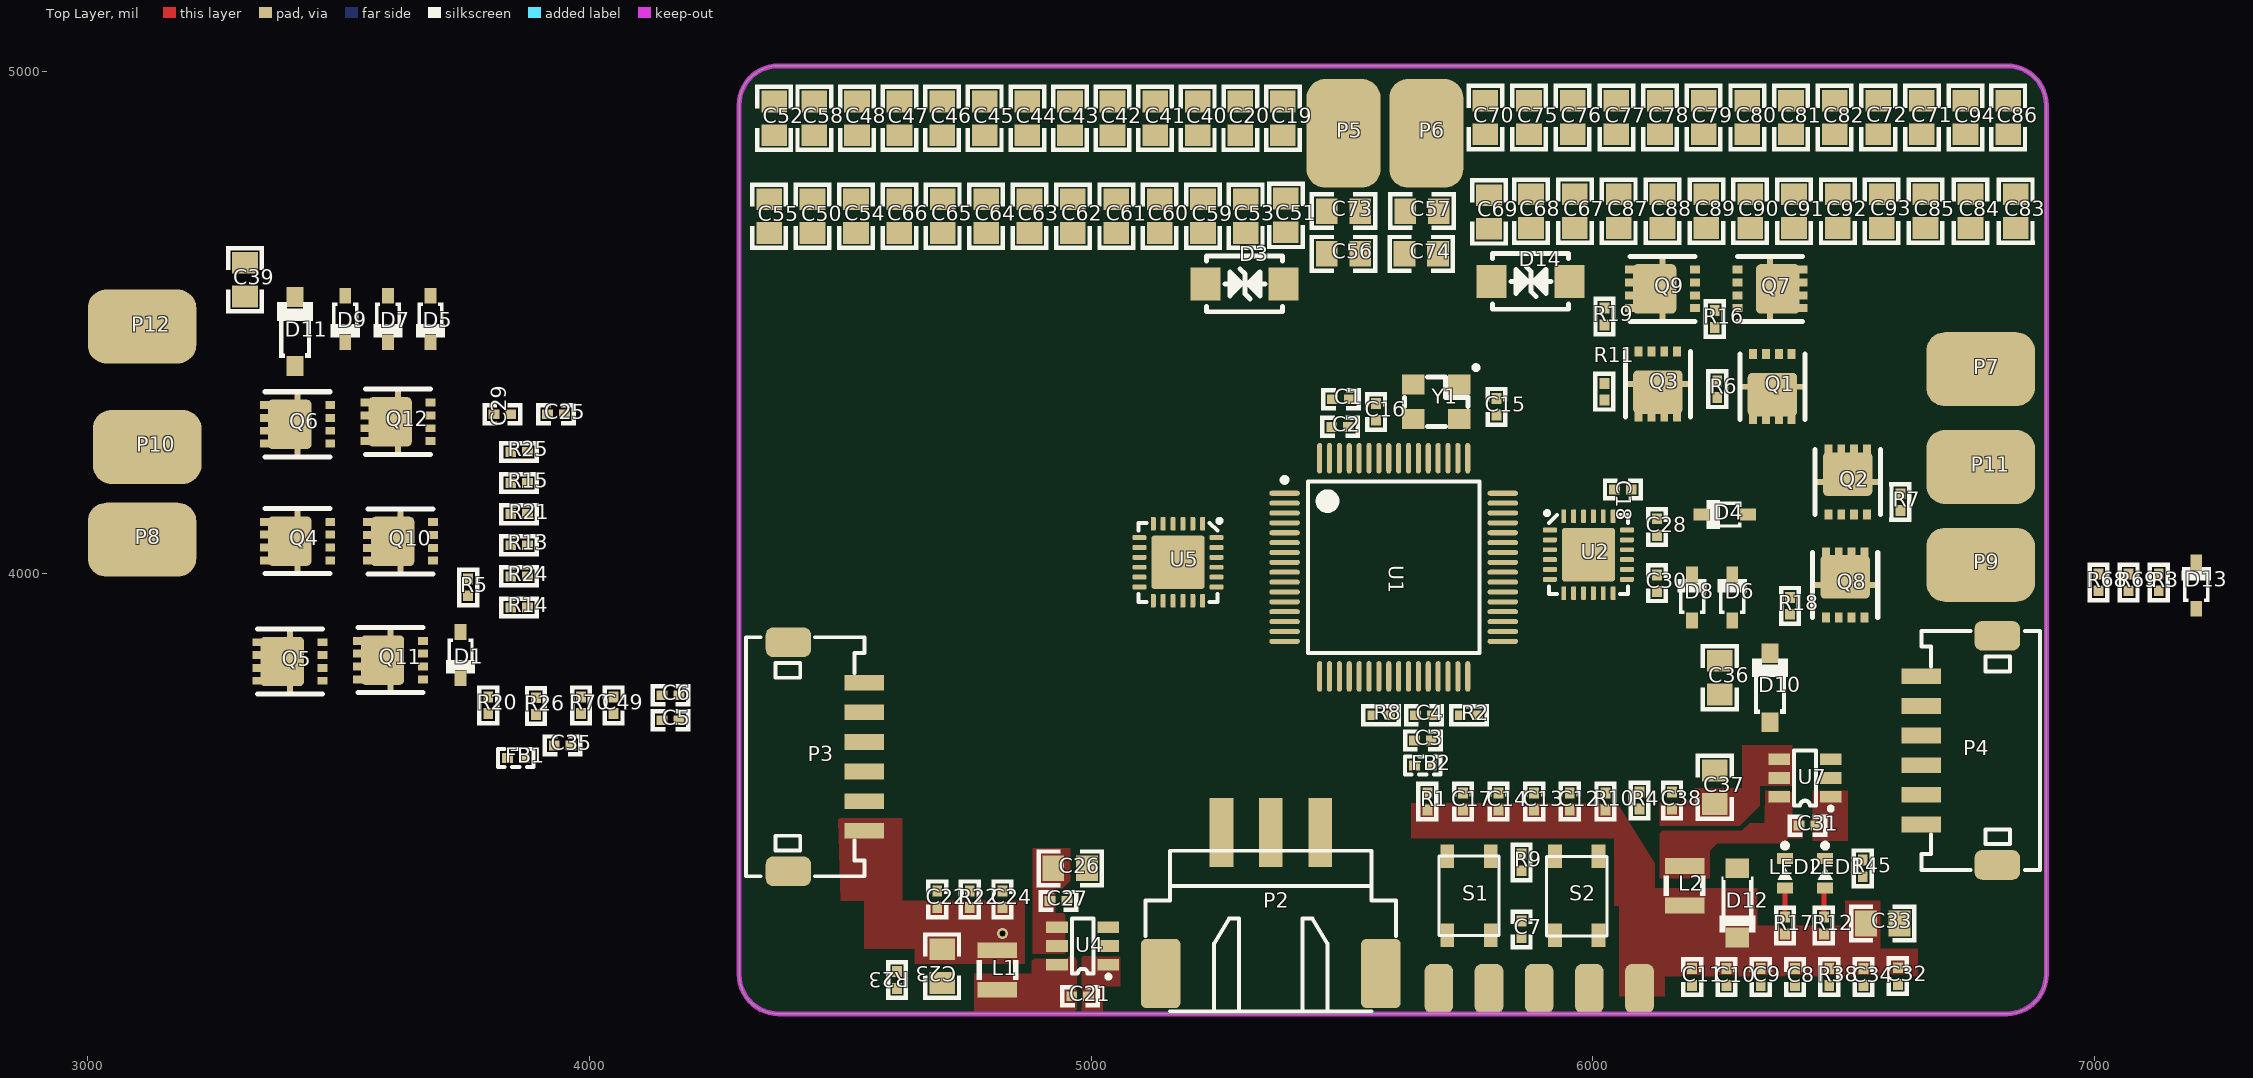
[diagram p0: Top Layer view]
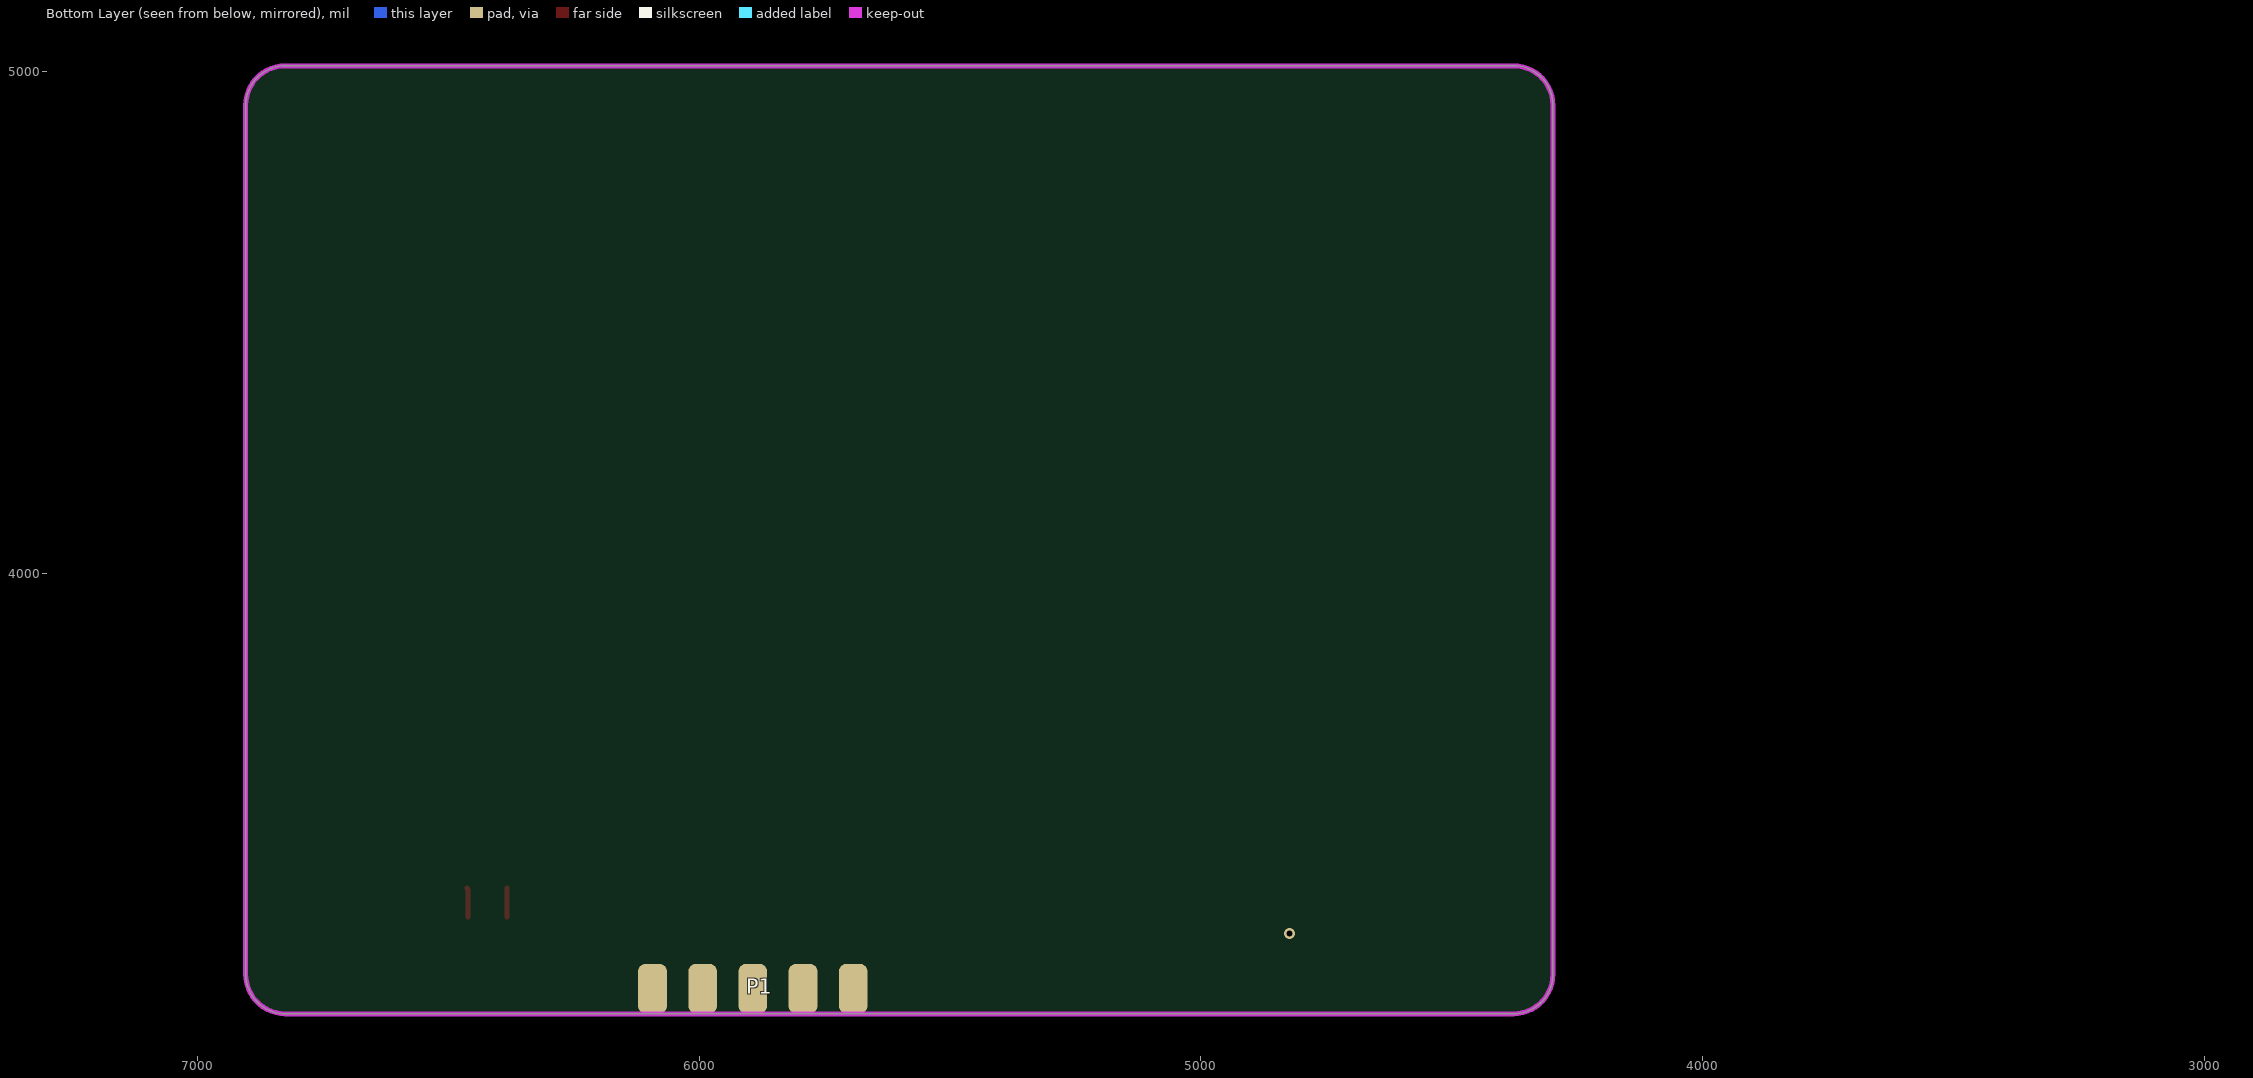
[diagram p1: Bottom Layer view, seen from below]
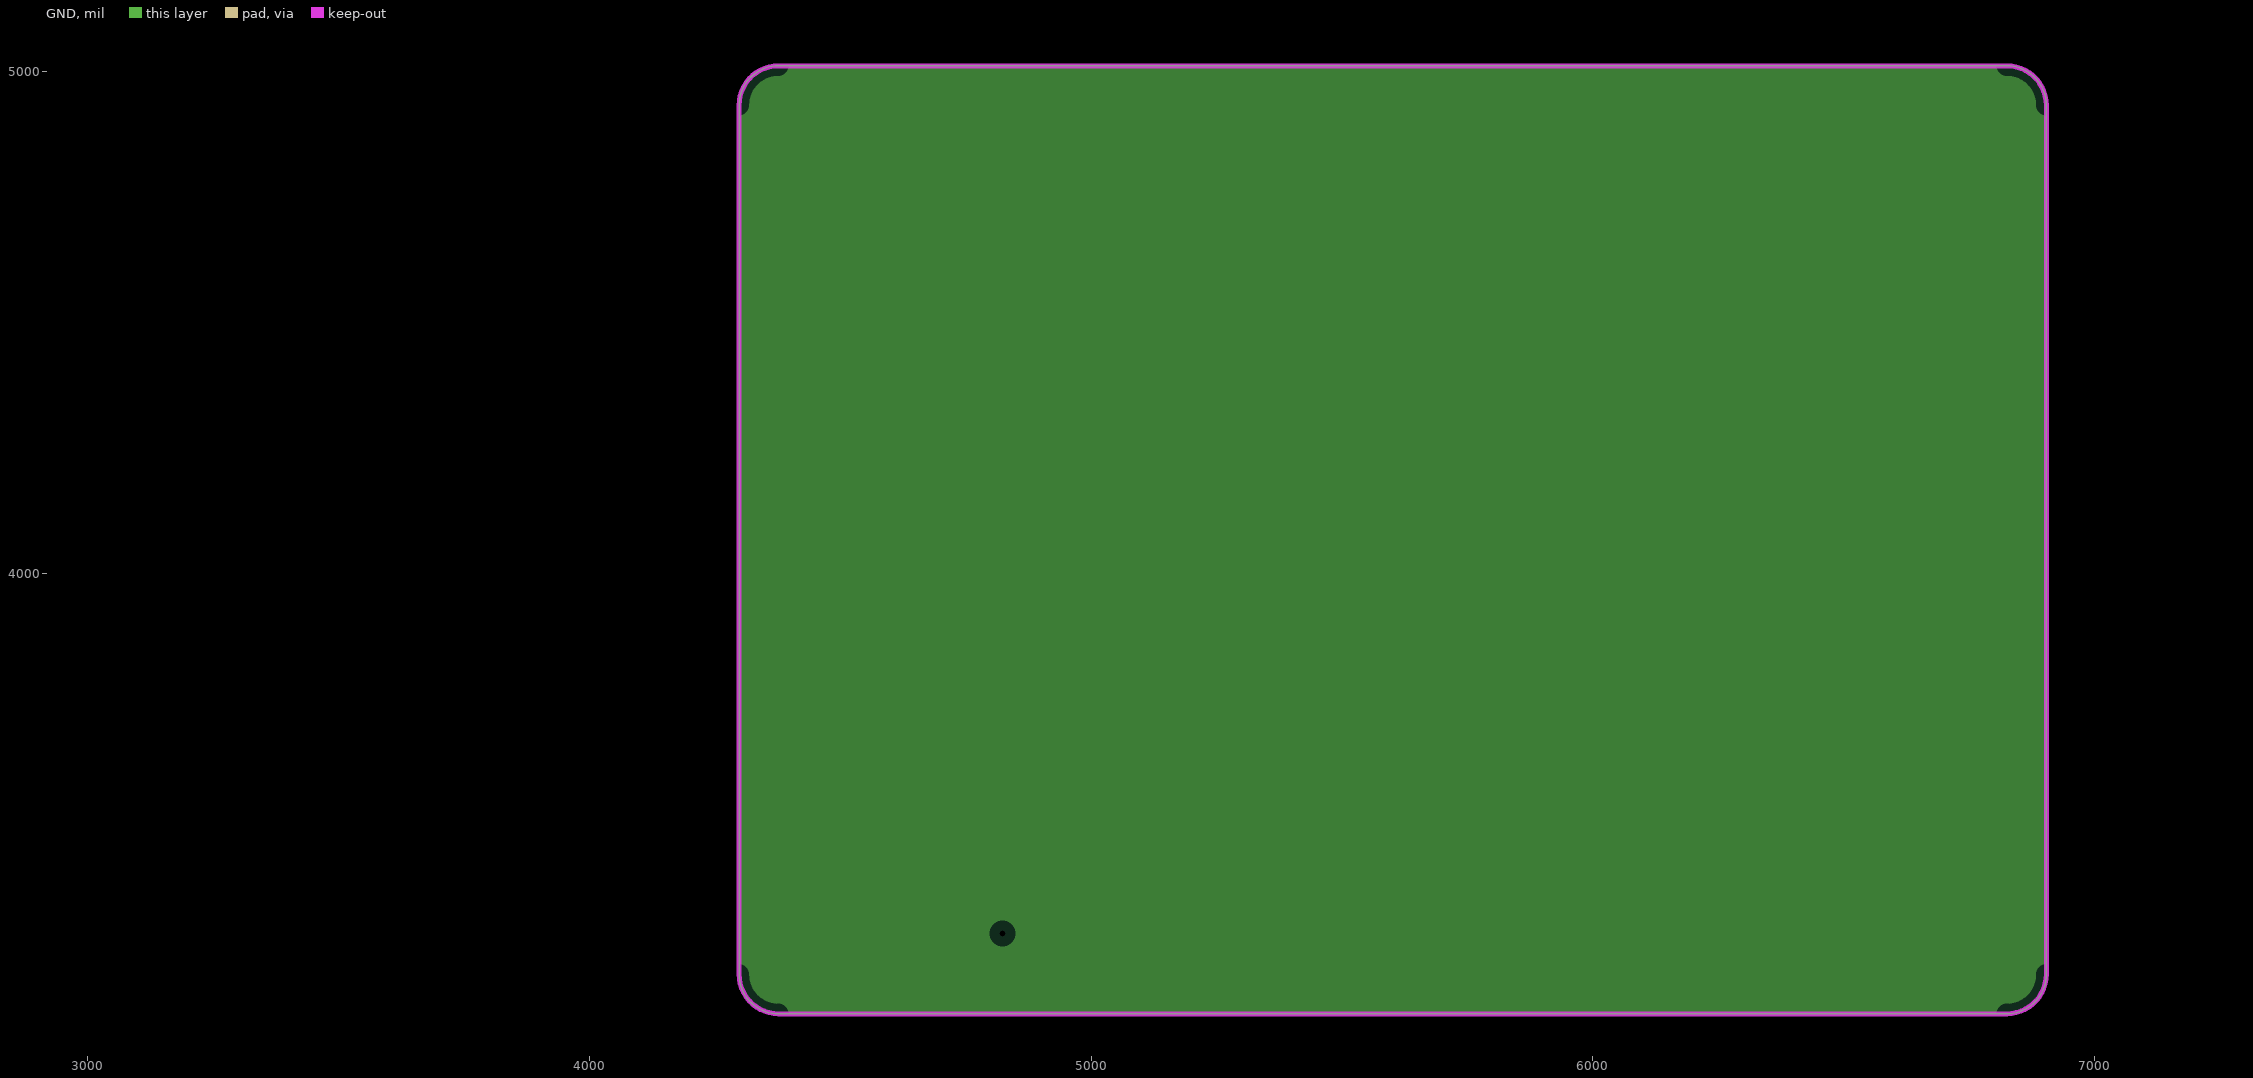
[diagram p2: GND, clearances drawn from the general rule]
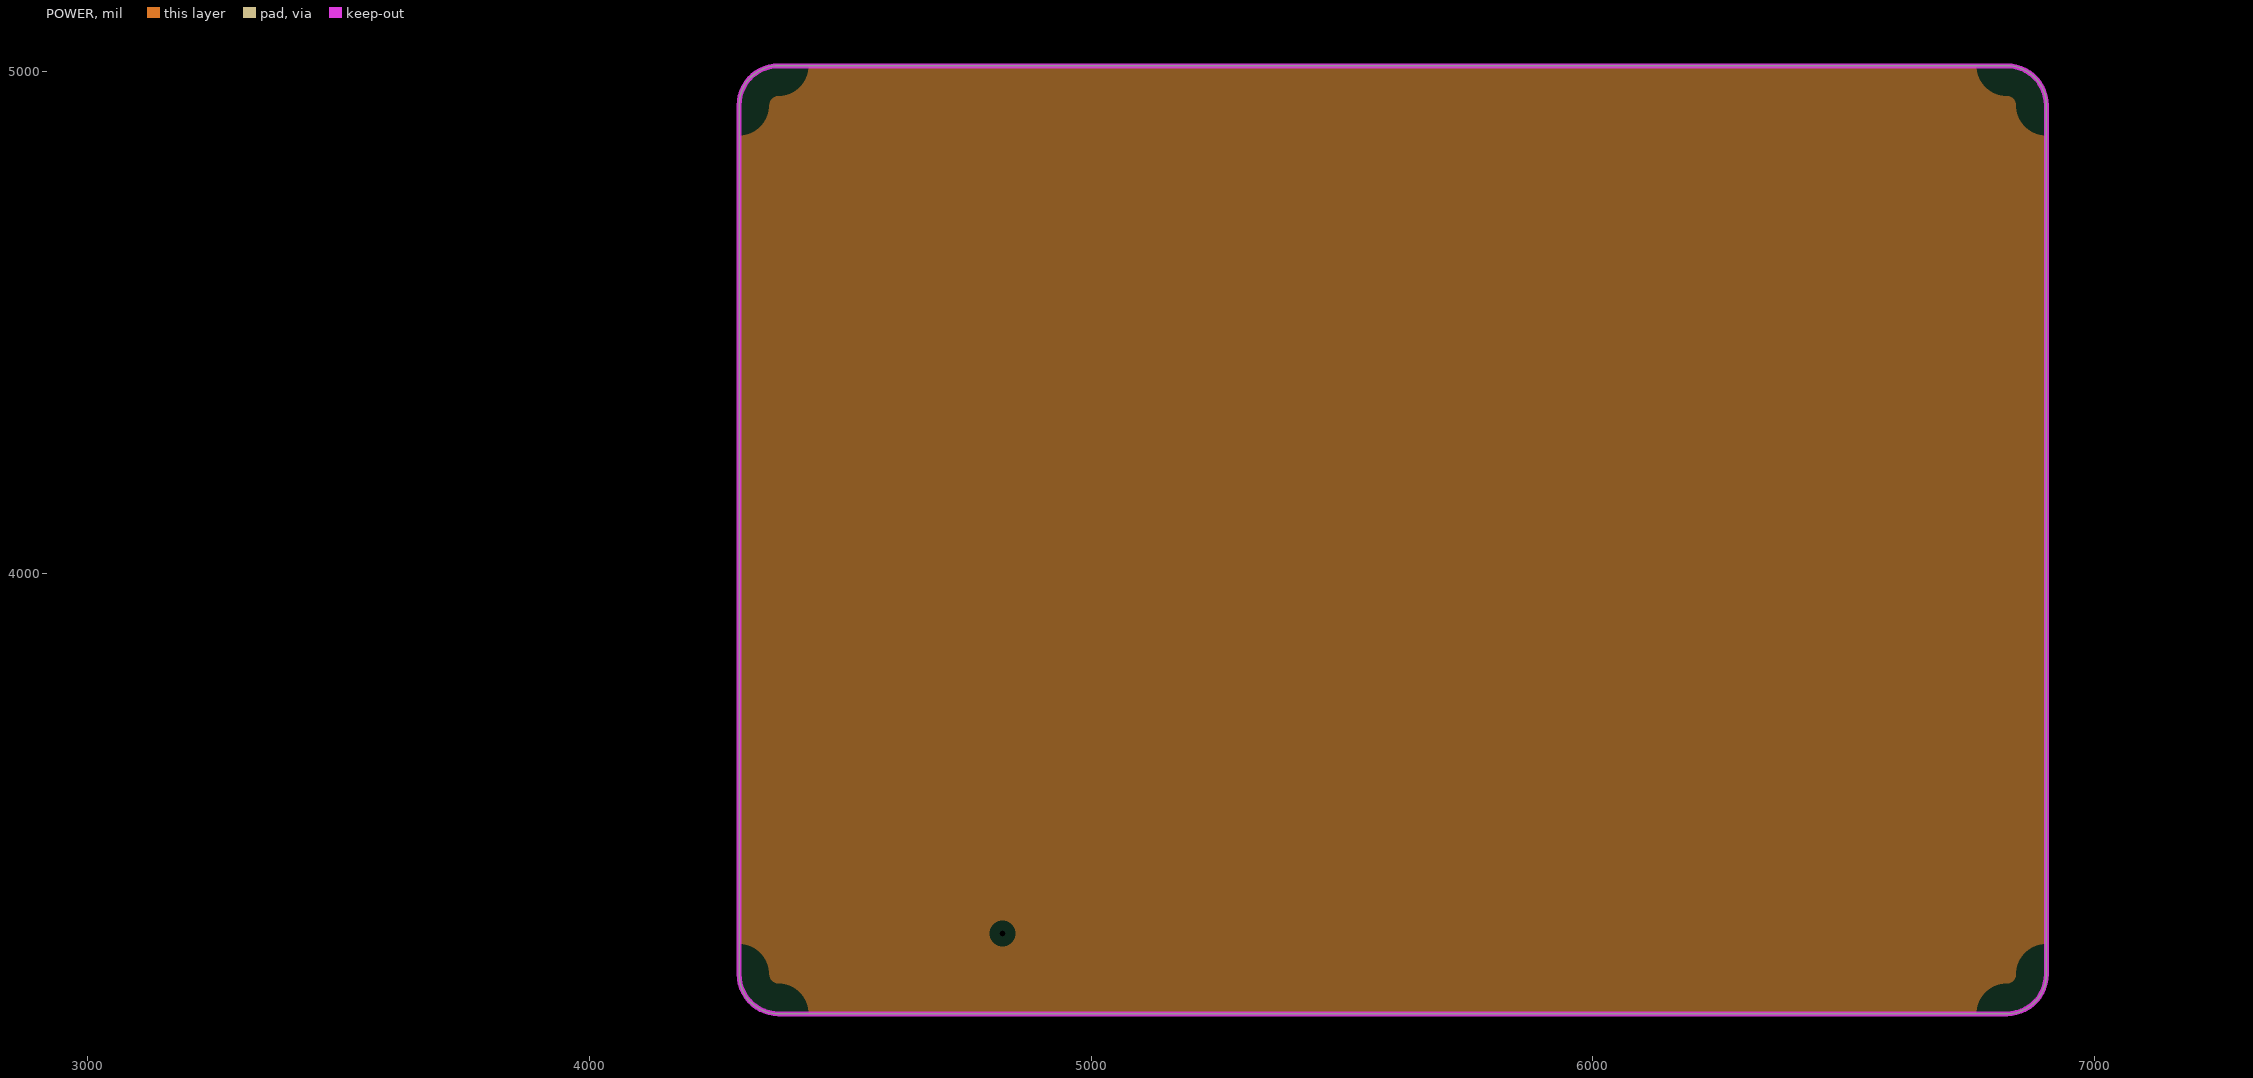
[diagram p3: POWER, clearances drawn from the general rule]
# Altium PCB MISC49862.pcbdoc
Units mil, origin at the board's own origin, x right, y up, seen from the top; angles counter-clockwise.
Board outline 2605.91 x 1889.76 mil, 4 copper layers (Top Layer, GND, POWER, Bottom Layer), stack 23.756 mil thick; 176 components, 102 nets, 585 pads, 1 vias.

## Layer stack, top to bottom
Top Solder Mask Layer: solder mask 0.4, Solder Resist, Dk 3.5
Top Layer: signal copper 1.4
Dielectric 3: surface 2.8, PP-006, Dk 4.1
GND: plane copper 1.378
Dielectric 2: surface 2.8, PP-006, Dk 4.1
POWER: plane copper 1.378
Dielectric 1: surface 12.6, FR-4, Dk 4.8
Bottom Layer: signal copper 1.4
Bottom Solder Mask Layer: solder mask 0.4, Solder Resist, Dk 3.5

## Board outline
6825.43,3122.38 4377.01,3122.38 cw(c4377.01,3201.12) 4298.27,3201.12 4298.27,4933.4 cw(c4377.01,4933.4) 4377.01,5012.14 6825.43,5012.14 cw(c6825.43,4933.4) 6904.17,4933.4 6904.17,3201.12 cw(c6825.43,3201.12)

## Design rules (kind name [scope] priority, off if disabled: settings)
HoleToHoleClearance Clearance_1 [All] p1 off: gap=11.8 allowstackedmicrovias=TRUE
HoleToHoleClearance Clearance [All] p2 off: gap=11.8 allowstackedmicrovias=TRUE
HoleToHoleClearance Width [All] p3 off: gap=120 allowstackedmicrovias=TRUE
HoleToHoleClearance DiffPairsRouting [All] p4 off: gap=15 allowstackedmicrovias=TRUE
HoleToHoleClearance RoutingVias [All] p5 off: gap=25 allowstackedmicrovias=TRUE
HoleToHoleClearance PlaneConnect [All] p6 off: gap=1 allowstackedmicrovias=TRUE
HoleToHoleClearance PolygonConnect [All] p7 off: gap=1 allowstackedmicrovias=TRUE
HoleToHoleClearance SolderMaskExpansion [All] p8 off: gap=4 allowstackedmicrovias=TRUE
HoleToHoleClearance PasteMaskExpansion [All] p9 off: gap=11.8 allowstackedmicrovias=TRUE
HoleToHoleClearance [All] p10: gap=10 allowstackedmicrovias=TRUE

## Components (designator, comment, footprint, x,y, rotation, side; value= is the part's Value field where it differs from the comment)
C1 "4.7uF 10V X5R" CAPC1005[0402]S-N 5498.27,4347.38 r0 top
C2 "100nF 16V X7R" CAPC1005[0402]S-N 5496.54,4292.38 r0 top
C3 "4.7uF 10V X5R" CAPC1005[0402]S-N 5661.54,3667.38 r180 top
C4 "100nF 16V X7R" CAPC1005[0402]S-N 5663.27,3717.38 r0 top
C5 "2.2uF 10V X5R" CAPC1005[0402]S-N 4161.54,3707.38 r0 top
C6 "100nF 16V X7R" CAPC1005[0402]S-N 4161.54,3757.38 r0 top
C7 "100nF 16V X7R" CAPC1005[0402]S-N 5858.27,3290.65 r270 top
C8 "4.7uF 10V X5R" CAPC1005[0402]S-N 6403.26,3195.65 r90 top
C9 "4.7uF 10V X5R" CAPC1005[0402]S-N 6334.93,3195.68 r270 top
C10 "100nF 16V X7R" CAPC1005[0402]S-N 6266.59,3195.65 r90 top
C11 "100nF 16V X7R" CAPC1005[0402]S-N 6198.27,3195.69 r270 top
C12 "4.7uF 10V X5R" CAPC1005[0402]S-N 5954.27,3545.65 r270 top
C13 "100nF 16V X7R" CAPC1005[0402]S-N 5883.27,3545.65 r270 top
C14 "4.7uF 10V X5R" CAPC1005[0402]S-N 5812.27,3545.65 r270 top
C15 "10pF 50V C0G" CAPC1005[0402]S-N 5808.27,4332.38 r270 top
C16 "10pF 50V C0G" CAPC1005[0402]S-N 5568.27,4322.38 r270 top
C17 "100nF 16V X7R" CAPC1005[0402]S-N 5741.27,3545.65 r270 top
C18 "4.7uF 10V X5R" CAPC1005[0402]S-N 6060,4167.38 r180 top
C19 "22uF 25V X5R" CAPC2012[0805]S-N 5382.43,4907.36 r90 top
C20 "22uF 25V X5R" CAPC2012[0805]S-N 5297.52,4907.38 r90 top
C21 "100nF 16V X7R" CAPC1005[0402]S-N 4978.27,3157.38 r180 top
C22 "220pF 50V X7R" CAPC1005[0402]S-N 4693.27,3350.65 r270 top
C23 "22uF 25V X5R" CAPC2012[0805]S-N 4703.27,3217.38 r90 top
C24 "100nF 16V X7R" CAPC1005[0402]S-N 4823.27,3350.65 r270 top
C25 "4.7uF 10V X5R" CAPC1005[0402]S-N 3933.27,4317.38 r0 top
C26 "22uF 25V X5R" CAPC2012[0805]S-N 4958.27,3412.38 r180 top
C27 "100nF 16V X7R" CAPC1005[0402]S-N 4935,3347.38 r180 top
C28 "4.7uF 10V X5R" CAPC1005[0402]S-N 6128.27,4092.38 r270 top
C29 "4.7uF 10V X5R" CAPC1005[0402]S-N 3826.54,4317.38 r0 top
C30 "4.7uF 10V X5R" CAPC1005[0402]S-N 6128.27,3980.65 r90 top
C31 "100nF 16V X7R" CAPC1005[0402]S-N 6428.27,3497.38 r180 top
C32 "220pF 50V X7R" CAPC1005[0402]S-N 6608.27,3197.38 r90 top
C33 "22uF 25V X5R" CAPC2012[0805]S-N 6578.27,3302.38 r180 top
C34 "100nF 16V X7R" CAPC1005[0402]S-N 6539.93,3195.65 r90 top
C35 "4.7uF 10V X5R" CAPC1005[0402]S-N 3946.54,3657.38 r0 top
C36 "22uF 25V X5R" CAPC2012[0805]S-N 6253.27,3792.38 r270 top
C37 "22uF 25V X5R" CAPC2012[0805]S-N 6243.27,3573.91 r270 top
C38 "100nF 16V X7R" CAPC1005[0402]S-N 6158.27,3547.38 r270 top
C39 "22uF 25V X5R" CAPC2012[0805]S-N 3313.27,4585.84 r90 top
C40 "22uF 25V X5R" CAPC2012[0805]S-N 5212.6,4907.36 r90 top
C41 "22uF 25V X5R" CAPC2012[0805]S-N 5127.68,4907.38 r90 top
C42 "22uF 25V X5R" CAPC2012[0805]S-N 5042.77,4907.36 r90 top
C43 "22uF 25V X5R" CAPC2012[0805]S-N 4957.85,4907.38 r90 top
C44 "22uF 25V X5R" CAPC2012[0805]S-N 4872.94,4907.37 r90 top
C45 "22uF 25V X5R" CAPC2012[0805]S-N 4788.02,4907.38 r90 top
C46 "22uF 25V X5R" CAPC2012[0805]S-N 4703.12,4907.36 r90 top
C47 "22uF 25V X5R" CAPC2012[0805]S-N 4618.18,4907.36 r90 top
C48 "22uF 25V X5R" CAPC2012[0805]S-N 4533.27,4907.36 r90 top
C49 "100nF 16V X7R" CAPC1005[0402]S-N 4048.27,3737.38 r270 top
C50 "22uF 25V X5R" CAPC2012[0805]S-N 4444.77,4712.38 r270 top
C51 "22uF 25V X5R" CAPC2012[0805]S-N 5388.27,4713.91 r270 top
C52 "22uF 25V X5R" CAPC2012[0805]S-N 4368.27,4907.38 r90 top
C53 "22uF 25V X5R" CAPC2012[0805]S-N 5308.27,4712.38 r270 top
C54 "22uF 25V X5R" CAPC2012[0805]S-N 4531.28,4712.38 r270 top
C55 "22uF 25V X5R" CAPC2012[0805]S-N 4358.27,4712.38 r270 top
C56 "22uF 25V X5R" CAPC2012[0805]S-N 5503.27,4637.38 r0 top
C57 "22uF 25V X5R" CAPC2012[0805]S-N 5659.8,4722.38 r180 top
C58 "22uF 25V X5R" CAPC2012[0805]S-N 4448.27,4907.36 r90 top
C59 "22uF 25V X5R" CAPC2012[0805]S-N 5223.27,4712.38 r270 top
C60 "22uF 25V X5R" CAPC2012[0805]S-N 5136.77,4712.38 r270 top
C61 "22uF 25V X5R" CAPC2012[0805]S-N 5050.28,4712.38 r270 top
C62 "22uF 25V X5R" CAPC2012[0805]S-N 4963.78,4712.38 r270 top
C63 "22uF 25V X5R" CAPC2012[0805]S-N 4877.28,4712.38 r270 top
C64 "22uF 25V X5R" CAPC2012[0805]S-N 4790.76,4712.38 r270 top
C65 "22uF 25V X5R" CAPC2012[0805]S-N 4704.28,4712.38 r270 top
C66 "22uF 25V X5R" CAPC2012[0805]S-N 4617.77,4712.38 r270 top
C67 "22uF 25V X5R" CAPC2012[0805]S-N 5964.5,4722.4 r90 top
C68 "22uF 25V X5R" CAPC2012[0805]S-N 5877.13,4722.35 r90 top
C69 "22uF 25V X5R" CAPC2012[0805]S-N 5793.27,4720.84 r90 top
C70 "22uF 25V X5R" CAPC2012[0805]S-N 5785.99,4908.91 r270 top
C71 "22uF 25V X5R" CAPC2012[0805]S-N 6656.24,4908.91 r270 top
C72 "22uF 25V X5R" CAPC2012[0805]S-N 6569.22,4908.91 r270 top
C73 "22uF 25V X5R" CAPC2012[0805]S-N 5503.27,4722.38 r180 top
C74 "22uF 25V X5R" CAPC2012[0805]S-N 5658.27,4637.38 r0 top
C75 "22uF 25V X5R" CAPC2012[0805]S-N 5873,4908.91 r270 top
C76 "22uF 25V X5R" CAPC2012[0805]S-N 5960.03,4908.91 r270 top
C77 "22uF 25V X5R" CAPC2012[0805]S-N 6047.06,4908.91 r270 top
C78 "22uF 25V X5R" CAPC2012[0805]S-N 6134.07,4908.91 r270 top
C79 "22uF 25V X5R" CAPC2012[0805]S-N 6221.11,4908.91 r270 top
C80 "22uF 25V X5R" CAPC2012[0805]S-N 6308.14,4908.91 r270 top
C81 "22uF 25V X5R" CAPC2012[0805]S-N 6395.16,4908.91 r270 top
C82 "22uF 25V X5R" CAPC2012[0805]S-N 6482.19,4908.91 r270 top
C83 "22uF 25V X5R" CAPC2012[0805]S-N 6843.27,4722.38 r90 top
C84 "22uF 25V X5R" CAPC2012[0805]S-N 6753.27,4722.38 r90 top
C85 "22uF 25V X5R" CAPC2012[0805]S-N 6663.27,4722.39 r90 top
C86 "22uF 25V X5R" CAPC2012[0805]S-N 6828.27,4908.91 r270 top
C87 "22uF 25V X5R" CAPC2012[0805]S-N 6051.83,4722.38 r90 top
C88 "22uF 25V X5R" CAPC2012[0805]S-N 6139.18,4722.37 r90 top
C89 "22uF 25V X5R" CAPC2012[0805]S-N 6226.52,4722.37 r90 top
C90 "22uF 25V X5R" CAPC2012[0805]S-N 6313.87,4722.38 r90 top
C91 "22uF 25V X5R" CAPC2012[0805]S-N 6401.22,4722.38 r90 top
C92 "22uF 25V X5R" CAPC2012[0805]S-N 6488.57,4722.38 r90 top
C93 "22uF 25V X5R" CAPC2012[0805]S-N 6575.92,4722.38 r90 top
C94 "22uF 25V X5R" CAPC2012[0805]S-N 6743.27,4908.9 r270 top
D1 "B5819WS" SOD-323 3743.27,3837.38 r270 top
D3 "SMAJ16CA" SMA[DO-214AC]-Bi 5305.93,4577.38 r180 top
D4 "B5819WS" SOD-323 6263.27,4117.38 r180 top
D5 "B5819WS" SOD-323 3683.27,4507.38 r270 top
D6 "B5819WS" SOD-323 6278.27,3952.38 r90 top
D7 "B5819WS" SOD-323 3598.27,4507.38 r270 top
D8 "B5819WS" SOD-323 6198.27,3952.38 r90 top
D9 "B5819WS" SOD-323 3513.27,4507.38 r270 top
D10 "BZT52C15" SOD-123-L 6353.27,3772.38 r90 top
D11 "BZT52C15" SOD-123-L 3413.27,4482.38 r90 top
D12 "SMF3.3A" SOD-123-FL 6288.27,3343.48 r270 top
D13 "B5819WS" SOD-323 7203.27,3976.12 r90 top
D14 "SMAJ16CA" SMA[DO-214AC]-Bi 5875.93,4582.38 r180 top
FB1 "120R @100MHz 500mA" INDC1005[0402]S 3853.27,3632.38 r0 top
FB2 "120R @100MHz 500mA" INDC1005[0402]S 5661.34,3617.38 r180 top
L1 "4.7uH 2A" SLO2520 4813.27,3209.57 r270 top
L2 "4.7uH 2A" SLO2520 6183.27,3377.38 r90 top
LED1 "Red SMD LED" LEDC1608(0603)-L 6463.27,3402.38 r270 top
LED2 "Blue SMD LED" LEDC1608(0603)-L 6383.27,3402.38 r270 top
P1 "SWD Header 5x2" HDR2X5-OB 5893.27,3172.38 r270 bottom
P2 "XH2.54-3P" XH2.54-3P-SH 5358.27,3287.38 r0 top
P3 "ZH1.5-6P" ZH1.5-6P-SH 4440,3634.74 r270 top
P4 "ZH1.5-6P" ZH1.5-6P-SH 6763.27,3647.38 r90 top
P5 "WirePad" WirePad-4x6 5503.27,4877.38 r90 top
P6 "WirePad" WirePad-4x6 5668.27,4877.38 r90 top
P7 "WirePad" WirePad-4x6 6773.27,4407.38 r0 top
P8 "WirePad" WirePad-4x6 3108.27,4067.38 r0 top
P9 "WirePad" WirePad-4x6 6773.27,4017.38 r0 top
P10 "WirePad" WirePad-4x6 3118.27,4252.38 r0 top
P11 "WirePad" WirePad-4x6 6773.27,4212.38 r0 top
P12 "WirePad" WirePad-4x6 3108.27,4492.38 r0 top
Q1 "TPN2R703NL" TSON3x3 6358.27,4372.38 r180 top
Q2 "TPN2R703NL" TSON3x3 6508.27,4182.38 r0 top
Q3 "TPN2R703NL" TSON3x3 6129.88,4377.42 r180 top
Q4 "TPN2R703NL" TSON3x3 3418.31,4064.58 r90 top
Q5 "TPN2R703NL" TSON3x3 3403.31,3824.58 r90 top
Q6 "TPN2R703NL" TSON3x3 3418.27,4297.38 r90 top
Q7 "TPN2R703NL" TSON3x3 6353.27,4567.38 r270 top
Q8 "TPN2R703NL" TSON3x3 6503.27,3977.38 r0 top
Q9 "TPN2R703NL" TSON3x3 6139.02,4567.38 r90 top
Q10 "TPN2R703NL" TSON3x3 3623.31,4063.99 r90 top
Q11 "TPN2R703NL" TSON3x3 3603.27,3827.38 r90 top
Q12 "TPN2R703NL" TSON3x3 3618.27,4302.38 r90 top
R1 "10K ±1%" RESC1005[0402]S-N 5670.3,3545.61 r90 top
R2 "0R ±1%" RESC1005[0402]S-N 5753.27,3717.38 r0 top
R3 "100R ±1%" RESC1005[0402]S-N 7128.27,3982.38 r90 top
R4 "100R ±1%" RESC1005[0402]S-N 6093.27,3547.38 r270 top
R5 "100R ±1%" RESC1005[0402]S-N 3758.27,3972.38 r270 top
R6 "4.7R ±1%" RESC1005[0402]S-N 6248.27,4367.38 r90 top
R7 "4.7R ±1%" RESC1005[0402]S-N 6613.27,4142.38 r270 top
R8 "0R ±1%" RESC1005[0402]S-N 5578.27,3717.38 r180 top
R9 "100R ±1%" RESC1005[0402]S-N 5858.27,3424.11 r270 top
R10 "4.7K ±1%" RESC1005[0402]S-N 6025.29,3545.61 r90 top
R11 "4.7R ±1%" RESC1005[0402]S-N 6023.27,4362.38 r90 top
R12 "1K ±1%" RESC1005[0402]S-N 6460.77,3298.32 r90 top
R13 "4.7R ±1%" RESC1005[0402]S-N 3860,4056.37 r180 top
R14 "4.7R ±1%" RESC1005[0402]S-N 3860,3932.38 r180 top
R15 "4.7R ±1%" RESC1005[0402]S-N 3860,4180.37 r180 top
R16 "4.7R ±1%" RESC1005[0402]S-N 6243.27,4507.38 r90 top
R17 "1K ±1%" RESC1005[0402]S-N 6383.27,3298.32 r90 top
R18 "4.7R ±1%" RESC1005[0402]S-N 6393.27,3935.65 r270 top
R19 "4.7R ±1%" RESC1005[0402]S-N 6023.27,4512.38 r90 top
R20 "100R ±1%" RESC1005[0402]S-N 3798.27,3737.37 r270 top
R21 "4.7R ±1%" RESC1005[0402]S-N 3860,4118.38 r180 top
R22 "73.2K ±1%" RESC1005[0402]S-N 4758.27,3350.65 r270 top
R23 "10K ±1%" RESC1005[0402]S-N 4613.27,3189.82 r270 top
R24 "4.7R ±1%" RESC1005[0402]S-N 3860,3994.38 r180 top
R25 "4.7R ±1%" RESC1005[0402]S-N 3860,4242.38 r180 top
R26 "100R ±1%" RESC1005[0402]S-N 3893.27,3735.65 r270 top
R38 "45.3K ±1%" RESC1005[0402]S-N 6471.63,3195.64 r90 top
R45 "10K ±1%" RESC1005[0402]S-N 6538.27,3412.38 r90 top
R68 "1K ±1%" RESC1005[0402]S-N 7008.27,3982.38 r90 top
R69 "10K ±1%" RESC1005[0402]S-N 7068.27,3982.38 r270 top
R70 "100R ±1%" RESC1005[0402]S-N 3983.27,3737.36 r90 top
S1 "KEY-TS1145" TS1145-B-A 5753.27,3357.38 r270 top
S2 "KEY-TS1145" TS1145-B-A 5968.27,3357.38 r90 top
U1 "CYT2BL3CAx" LQFP64_L 5603.27,4012.38 r0 top
U2 "FD6288Q" QFN24-4x4-L 5991.5,4037.54 r0 top
U4 "RY9121E" SOT-23-6 4983.27,3257.38 r180 top
U5 "FD6288Q" QFN24-4x4-L 5173.27,4022.38 r270 top
U7 "RY9121E" SOT-23-6 6423.27,3592.38 r180 top
Y1 "16MHz 20pF" X3225-4 5688.27,4342.38 r180 top

## Footprints (in the part's own frame and the unit in brackets; to place one, negate y for a bottom-side part, rotate by r counter-clockwise, add the part's x,y. Pads: shape width x height; smd on the part's side, far side on the other; paste and mask are expansions set on the pad)
CAPC1005[0402]S-N [mm]
  rect 0.55x0.5 smd: 1(-0.425,0) 2(0.425,0)
  silkscreen extent -1,-0.55 1,0.55
CAPC2012[0805]S-N [mm]
  rect 1.1x1.3 smd: 1(-0.85,0) 2(0.85,0)
  silkscreen extent -1.7,-0.95 1.7,0.95
HDR2X5-OB [mm]
  rrect50% 2.5x1.45 smd paste+0 mask+0.01: 1(0,5.08) 3(0,2.54) 5(0,0) 7(0,-2.54) 9(0,-5.08)
  rrect50% 2.5x1.45 smd far side paste+0 mask+0.01: 2(0,5.08) 4(0,2.54) 6(0,0) 8(0,-2.54) 10(0,-5.08)
INDC1005[0402]S [mm]
  rect 0.55x0.5 smd: 1(-0.43,0) 2(0.43,0)
  silkscreen extent -0.9,-0.45 0.9,0.45
LEDC1608(0603)-L [mm]
  rect 0.55x0.8 smd: A(0.75,0) C(-0.75,0)
  silkscreen extent -1.52,-0.38 0.33,0.38
LQFP64_L [mm]
  oval 1.55x0.254 smd: 1(-5.525,3.75) 2(-5.525,3.25) 3(-5.525,2.75) 4(-5.525,2.25) 5(-5.525,1.75) 6(-5.525,1.25) 7(-5.525,0.75) 8(-5.525,0.25) 9(-5.525,-0.25) 10(-5.525,-0.75) 11(-5.525,-1.25) 12(-5.525,-1.75) 13(-5.525,-2.25) 14(-5.525,-2.75) 15(-5.525,-3.25) 16(-5.525,-3.75) 33(5.525,-3.75) 34(5.525,-3.25) 35(5.525,-2.75) 36(5.525,-2.25) 37(5.525,-1.75) 38(5.525,-1.25) 39(5.525,-0.75) 40(5.525,-0.25) 41(5.525,0.25) 42(5.525,0.75) 43(5.525,1.25) 44(5.525,1.75) 45(5.525,2.25) 46(5.525,2.75) 47(5.525,3.25) 48(5.525,3.75)
  oval 0.254x1.55 smd: 17(-3.75,-5.525) 18(-3.25,-5.525) 19(-2.75,-5.525) 20(-2.25,-5.525) 21(-1.75,-5.525) 22(-1.25,-5.525) 23(-0.75,-5.525) 24(-0.25,-5.525) 25(0.25,-5.525) 26(0.75,-5.525) 27(1.25,-5.525) 28(1.75,-5.525) 29(2.25,-5.525) 30(2.75,-5.525) 31(3.25,-5.525) 32(3.75,-5.525) 49(3.75,5.525) 50(3.25,5.525) 51(2.75,5.525) 52(2.25,5.525) 53(1.75,5.525) 54(1.25,5.525) 55(0.75,5.525) 56(0.25,5.525) 57(-0.25,5.525) 58(-0.75,5.525) 59(-1.25,5.525) 60(-1.75,5.525) 61(-2.25,5.525) 62(-2.75,5.525) 63(-3.25,5.525) 64(-3.75,5.525)
  silkscreen extent -5.65,-4.35 4.35,4.55
QFN24-4x4-L [mm]
  rrect50% 0.7x0.25 smd paste+0.102 mask+0.05: 1(-1.95,1.25) 2(-1.95,0.75) 3(-1.95,0.25) 4(-1.95,-0.25) 5(-1.95,-0.75) 6(-1.95,-1.25) 13(1.95,-1.25) 14(1.95,-0.75) 15(1.95,-0.25) 16(1.95,0.25) 17(1.95,0.75) 18(1.95,1.25)
  rrect50% 0.25x0.7 smd paste+0.102 mask+0.05: 7(-1.25,-1.95) 8(-0.75,-1.95) 9(-0.25,-1.95) 10(0.25,-1.95) 11(0.75,-1.95) 12(1.25,-1.95) 19(1.25,1.95) 20(0.75,1.95) 21(0.25,1.95) 22(-0.25,1.95) 23(-0.75,1.95) 24(-1.25,1.95)
  rrect10% 2.7x2.7 smd paste+0.102 mask+0.05: 25(0,0)
  silkscreen extent -2.2,-2 2,2.2
RESC1005[0402]S-N [mm]
  rect 0.55x0.5 smd: 1(-0.425,0) 2(0.425,0)
  silkscreen extent -1,-0.55 1,0.55
SLO2520 [mm]
  rect 0.8x2 smd: 1(-1,0) 2(1,0)
  silkscreen extent -0.5,-1.05 0.5,1.05
SMA[DO-214AC]-Bi [mm]
  rect 1.52x1.68 smd: A(-1.972,0) K(1.973,0)
  silkscreen extent -1.93,-1.41 1.93,1.41
SOD-123-FL [mm]
  rect 1x1.2 smd: A(-1.75,0) K(1.75,0)
  silkscreen extent -1.33,-0.9 1.5,0.9
SOD-123-L [mm]
  rect 1x0.85 smd: A(-1.75,0) K(1.75,0)
  silkscreen extent -1.32,-0.9 1.48,0.9
SOD-323 [mm]
  rect 0.8x0.6 smd: A(-1.175,0) K(1.175,0)
  silkscreen extent -0.83,-0.73 0.92,0.72
SOT-23-6 [mm]
  rect 1.1x0.6 smd: 1(-1.3,0.95) 2(-1.3,0) 3(-1.3,-0.95) 4(1.3,-0.95) 5(1.3,0) 6(1.3,0.95)
  silkscreen extent -1.37,-1.4 0.55,1.62
TS1145-B-A [mm]
  rect 1.2x0.7 smd: 1(-2,-1.1) 1(2,-1.1) 2(-2,1.1) 2(2,1.1)
  silkscreen extent -2.02,-1.52 2,1.52
TSON3x3 [mm]
  rect 0.4x0.5 smd: 1(-0.975,1.65) 1(-0.325,1.65) 1(0.325,1.65) 1(0.975,1.65) 2(0.975,-1.65) 3(-0.975,-1.65) 3(-0.325,-1.65) 3(0.325,-1.65)
  rrect20% 2.5x2.2 smd: 1(0,0.4)
  rrect20% 3.4x0.3 smd: 1(0,0)
  silkscreen extent -1.65,-1.65 1.65,1.65
WirePad-4x6 [mm]
  rrect50% 5.5x3.75 smd paste+0 mask+0.05: 1(0,0)
X3225-4 [mil]
  rect 45x39.37 smd: 1(-46,-34.4) 2(46,-34.41) 3(46,34.41) 4(-46,34.41)
  silkscreen extent -83,-72 63,49
XH2.54-3P-SH [mm]
  rrect25% 2x3.5 smd: 0(-5.577,-2.15) 0(5.577,-2.15)
  rect 1.2x3.5 smd: 1(-2.5,4.981) 2(0,4.981) 3(2.5,4.981)
  silkscreen extent -6.35,-4.06 6.35,4.06
ZH1.5-6P-SH [mm]
  rrect50% 1.5x2.3 smd: 0(-5.8,-1.1) 0(5.8,-1.1)
  rect 0.8x2 smd: 1(-3.75,2.75) 2(-2.25,2.75) 3(-0.75,2.75) 4(0.75,2.75) 5(2.25,2.75) 6(3.75,2.75)
  silkscreen extent -6.05,-3.25 6.05,2.75

## Via types
v1: diameter 22, hole 12, Top Layer to Bottom Layer, 1 vias

## Nets (pads, with @x,y where several pads share a name; then routed paths per layer and width w, separated by ;. In a path a pad name is that pad's centre, name@x,y a point inside that pad or via, vN(x,y) a via of type N, cw(c..) or ccw(c..) an arc to the next point about the centre after c; other vN are vias at no path point)
BATADC: R70.2 U1.20
DBG_RX: P1.2 U1.1
DBG_TX: P1.4 U1.2
ECD1_CS: P3.2 U1.12
ECD1_MISO: P3.3 U1.9
ECD1_MOSI: P3.4 U1.10
ECD1_SCLK: P3.5 U1.11
ECD2_CS: P4.2 U1.37
ECD2_MISO: P4.3 U1.34
ECD2_MOSI: P4.4 U1.35
ECD2_SCLK: P4.5 U1.36
ECO_IN: C15.1 U1.52 Y1.1
ECO_OUT: C16.2 U1.53 Y1.3
GND: C1.1 C2.1 C7.1 C8.1 C9.2 C10.1 C11.2 C12.1 C13.1 C14.1 C15.2 C16.1 C17.1 C19.2 C20.2 C22.1 C23.1 C24.1 C26.1 C27.1 C32.1 C33.1 C34.1 C36.2 C37.1 C38.1 C39.2 C40.2 C41.2 C42.2 C43.2 C44.2 C45.2 C46.2 C47.2 C48.2 C49.1 C50.2 C51.2 C52.2 C53.2 C54.2 C55.2 C56.2 C57.2 C58.2 C59.2 C60.2 C61.2 C62.2 C63.2 C64.2 C65.2 C66.2 C67.1 C68.1 C69.1 C70.1 C71.1 C72.1 C73.1 C74.1 C75.1 C76.1 C77.1 C78.1 C79.1 C80.1 C81.1 C82.1 C83.1 C84.1 C85.1 C86.1 C87.1 C88.1 C89.1 C90.1 C91.1 C92.1 C93.1 C94.1 D3.K D10.A D11.A D12.A D14.A FB2.1 LED1.C P1.6 P1.8 P2.3 P3.1 P4.1 P6.1 Q8.3 Q11.3 R22.1 R23.1 R23.2 R38.1 R45.1 R45.2 R68.1 S1.1 S2.1 U1.17 U1.33 U1.49 U1.56 U1.57 U2.6 U2.25 U4.2 U4.3 U5.6 U5.25 U7.2 U7.3 Y1.2 Y1.4
HOA1: R6.1 U2.19
HOA2: R13.1 U5.19
HOB1: R7.1 U2.16
HOB2: R14.1 U5.16
HOC1: R11.1 U2.13
HOC2: R15.1 U5.13
KEYMOD: R9.1 U1.15
LEDMOD: LED2.C U1.14
LOA1: R16.1 U2.11
LOA2: R21.1 U5.11
LOB1: R18.1 U2.10
LOB2: R24.1 U5.10
LOC1: R19.1 U2.9
LOC2: R25.1 U5.9
NETC21_1: C21.1 U4.1
NETC21_2: C21.2 L1.2 U4.6
NETC26_2: C26.2 C27.2 D1.K U4.4 U4.5
NETC31_1: C31.1 U7.1
NETC31_2: C31.2 L2.2 U7.6
NETC36_1: C36.1 D4.A D6.A D8.A D10.K R3.2 U2.4
NETC37_2: C37.2 C38.2 D13.K U7.4 U7.5
NETC39_1: C39.1 D5.A D7.A D9.A D11.K R5.2 U5.4
NETC49_2: C49.2 R70.1
NETLED1_A: LED1.A R12.2 | length 58.8
  Top Layer w10: R12.2 6460.77,3370.36 LED1.A
NETLED2_A: LED2.A R17.2 | length 57.8
  Top Layer w10: R17.2 LED2.A
NETP2_1: P2.1 R20.2
NETP2_2: P2.2 R26.2
NETQ1_1: Q1.1 Q3.1
NETQ1_2: Q1.2 R6.2
NETQ1_3: Q1.3 Q7.1
NETQ2_2: Q2.2 R7.2
NETQ3_2: Q3.2 R11.2
NETQ3_3: Q3.3 Q9.1
NETQ4_1: Q4.1 Q6.1
NETQ4_2: Q4.2 R13.2
NETQ4_3: Q4.3 Q10.1
NETQ5_2: Q5.2 R14.2
NETQ5_3: Q5.3 Q11.1
NETQ6_2: Q6.2 R15.2
NETQ6_3: Q6.3 Q12.1
NETQ7_2: Q7.2 R16.2
NETQ7_3: Q7.3 Q9.3
NETQ8_2: Q8.2 R18.2
NETQ9_2: Q9.2 R19.2
NETQ10_2: Q10.2 R21.2
NETQ10_3: Q10.3 Q12.3
NETQ11_2: Q11.2 R24.2
NETQ12_2: Q12.2 R25.2
NETR4_1: R4.1 U1.54
NETR9_2: R9.2 R10.2 S2.2
NETR68_2: R68.2 R69.1
PWM1AH: U1.38 U2.22
PWM1AL: U1.39 U2.1
PWM1BH: U1.44 U2.23
PWM1BL: U1.45 U2.2
PWM1CH: U1.46 U2.24
PWM1CL: U1.47 U2.3
PWM2AH: U1.3 U5.22
PWM2AL: U1.4 U5.1
PWM2BH: U1.5 U5.23
PWM2BL: U1.6 U5.2
PWM2CH: U1.7 U5.24
PWM2CL: U1.8 U5.3
RST: C7.2 P1.1 R1.2 R4.2 S1.2
SWCLK: P1.7 U1.62
SWDIO: P1.9 U1.63
UART_RX: R20.1 U1.18
UART_TX: R26.1 U1.19
VBA1: C18.2 D4.K U2.20
VBA2: C25.2 D5.K U5.20
VBAT: C19.1 C20.1 C40.1 C41.1 C42.1 C43.1 C44.1 C45.1 C46.1 C47.1 C48.1 C50.1 C51.1 C52.1 C53.1 C54.1 C55.1 C56.1 C57.1 C58.1 C59.1 C60.1 C61.1 C62.1 C63.1 C64.1 C65.1 C66.1 C67.2 C68.2 C69.2 C70.2 C71.2 C72.2 C73.2 C74.2 C75.2 C76.2 C77.2 C78.2 C79.2 C80.2 C81.2 C82.2 C83.2 C84.2 C85.2 C86.2 C87.2 C88.2 C89.2 C90.2 C91.2 C92.2 C93.2 C94.2 D1.A D3.A D13.A D14.K P5.1 Q2.1 Q5.1 R3.1 R5.1 R69.2
VBB1: C28.2 D6.K U2.17
VBB2: C29.2 D7.K U5.17
VBC1: C30.2 D8.K U2.14
VBC2: C35.2 D9.K U5.14
VCC1V1: C1.2 C2.2 U1.58
VCC3V3: C8.2 C9.1 C10.2 C11.1 C12.2 C13.2 C14.2 C17.2 C32.2 C33.2 C34.2 D12.K FB1.1 L2.1 P1.10 R1.1 R10.1 R12.1 R17.1 R38.2 U1.16 U1.32 U1.48 U1.55
VCC5V: C22.2 C23.2 C24.2 L1.1 P3.6 P4.6 R22.2
  other v1: 4823.27,3282.38
VDDA: C3.1 C4.2 FB1.2 R2.1 U1.28
VREFH: C5.2 C6.2 R2.2 U1.29
VREFL: C5.1 C6.1 R8.2 U1.26
VSA1: C18.1 P7.1 U2.18
VSA2: C25.1 P8.1 U5.18
VSB1: C28.1 P9.1 Q2.3 Q8.1 U2.15
VSB2: C29.1 P10.1 U5.15
VSC1: C30.1 P11.1 U2.12
VSC2: C35.1 P12.1 U5.12
VSSA: C3.2 C4.1 FB2.2 R8.1 U1.27
pads on no net: P1.3 P1.5 P2.0 P3.0 P4.0 U1.13 U1.21 U1.22 U1.23 U1.24 U1.25 U1.30 U1.31 U1.40 U1.41 U1.42 U1.43 U1.50 U1.51 U1.59 U1.60 U1.61 U1.64 U2.5 U2.7 U2.8 U2.21 U5.5 U5.7 U5.8 U5.21

## Polygon pours and split planes (outlines as drawn)
NETC26_2 on Top Layer (solid, pour order 26): 4883.27,3457.38 4958.27,3457.38 4958.27,3387.38 4943.27,3372.38 4928.27,3372.38 4928.27,3322.38 4948.27,3322.38 4948.27,3242.38 4883.27,3242.38
VCC5V on Top Layer (solid, pour order 0): 4495.54,3512.38 4623.27,3512.38 4623.27,3347.38 4868.27,3347.38 4868.27,3222.38 4648.27,3222.38 4648.27,3252.38 4548.27,3252.38 4548.27,3347.38 4500.54,3347.38
NETC31_1 on Top Layer (solid, pour order 42): 6438.27,3567.38 6508.27,3567.38 6508.27,3467.38 6438.27,3467.38
NETC31_2 on Top Layer (solid, pour order 40): 6133.27,3392.38 6233.27,3392.38 6233.27,3447.38 6248.27,3462.38 6388.27,3462.38 6388.27,3502.38 6308.27,3502.38 6293.27,3487.38 6133.27,3487.38
NETC31_2 on Top Layer (solid, pour order 38): 6343.27,3572.38 6393.27,3572.38 6398.27,3567.38 6398.27,3517.38 6418.27,3517.38 6418.27,3472.38 6343.27,3472.38
NETC37_2 on Top Layer (solid, pour order 36): 6398.27,3657.38 6398.27,3577.38 6333.27,3577.38 6333.27,3537.38 6293.27,3497.38 6133.27,3497.38 6133.27,3542.38 6138.27,3547.38 6203.27,3547.38 6203.27,3572.38 6298.27,3572.38 6298.27,3657.38
NETC21_1 on Top Layer (solid, pour order 30): 5058.27,3237.38 5058.27,3177.38 5023.27,3177.38 5023.27,3127.38 4978.27,3127.38 4978.27,3237.38
NETC21_2 on Top Layer (solid, pour order 28): 4766.8,3202.38 4881.8,3202.38 4881.8,3237.38 4971.8,3237.38 4971.8,3187.38 4971.8,3127.38 4766.8,3127.38
VCC3V3 on Top Layer (solid, pour order 22): 5638.27,3542.38 6048.27,3542.38 6123.27,3422.38 6123.27,3337.38 6043.27,3337.38 6043.27,3472.38 5638.27,3472.38
VCC3V3 on Top Layer (solid, pour order 16): 6053.27,3157.38 6143.27,3157.38 6143.27,3197.38 6648.27,3197.38 6648.27,3252.38 6573.27,3252.38 6573.27,3347.38 6513.27,3347.38 6503.27,3347.38 6503.27,3297.38 6328.27,3297.38 6328.27,3372.38 6053.27,3372.38

## Keep-outs
Board Outline Layer:
  the board outline again, w10

## Other copper
GND (plane layer: these items are gaps in the copper):
  the board outline again, w40
POWER (plane layer: these items are gaps in the copper):
  the board outline again, w120

## Silkscreen, mask and mechanical layers (free items; w line width, h text height)
Mechanical Layer:
  circle w0.5: c4475.24,3279.86 r66.93
  circle w0.5: c6727.2,3279.86 r66.93
  lines w0.5: 4298.27,3201.12 4298.27,4933.4 cw(c4377.01,4933.4) 4377.01,5012.14 6825.43,5012.14 cw(c6825.43,4933.4) 6904.17,4933.4 6904.17,3201.12 cw(c6825.43,3201.12) 6825.43,3122.38 4377.01,3122.38 cw(c4377.01,3201.12) 4298.27,3201.12